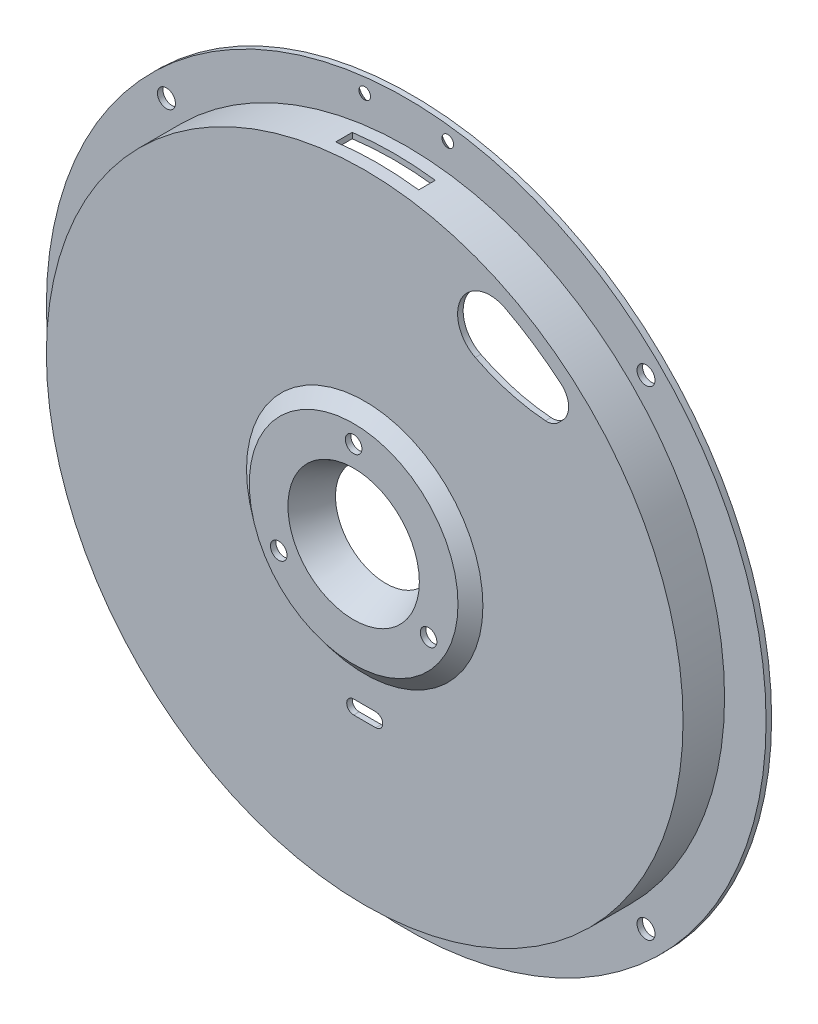
from build123d import *

# Parameters (mm, degrees)
CUT_EXTRUDE1_DEPTH                                   = 45
CUT_EXTRUDE2_DEPTH                                   = 10
SKETCH5_W                                            = 30
SKETCH5_H                                            = 6
CUT_EXTRUDE3_DEPTH                                   = 32
HOLE_SIZE_BY_CROSS_RECESS_COUNTERSUNK_SE_D           = 3.7
HOLE_SIZE_BY_CROSS_RECESS_COUNTERSUNK_SE_CSINK_D     = 8.2
HOLE_SIZE_BY_CROSS_RECESS_COUNTERSUNK_SE_CSINK_ANGLE = 90
SKETCH8_R                                            = 3.25
CUT_EXTRUDE4_DEPTH                                   = 186.04323819
CIRPATTERN1_COUNT                                    = 4
SKETCH9_R                                            = 3
CUT_EXTRUDE5_DEPTH                                   = 28
CIRPATTERN2_COUNT                                    = 3


with BuildPart() as part:
    # Sketch1 → Revolve1 (revolve)
    with BuildSketch(Plane(origin=(0, 0, 0), x_dir=(1, 0, 0), z_dir=(0, 1, 0)), mode=Mode.PRIVATE) as revolve1_sk:
        Polygon((-115, 15), (-130, 15), (-130, 17), (-113, 17), (-113, 2), (-67.400598844, 2), (-42, 2), (-37, -2), (-25, -2), (-20, 8.5), (-18.194278962, 7.640132839), (-23.737199362, -4), (-37.701562119, -4), (-42.701562119, 0), (-115, 0), align=None)
    revolve(revolve1_sk.sketch.rotate(Axis((0, 0, 0), (0, 0, -1)), 180), axis=Axis((0, 0, 0), (0, 0, -1)))

    # Sketch3 → Cut-Extrude1 (cut)
    with BuildSketch(Plane(origin=(0, 0, -17), x_dir=(-1, 0, 0), z_dir=(0, 0, -1))):
        with BuildLine():
            Line((-69.977392836, 70.947139279), (-71.467016668, 72.43676311))
            ThreePointArc((-71.467016668, 72.43676311), (-73.65767572, 78.041003905), (-71.024689008, 83.451538346))
            ThreePointArc((-71.024689008, 83.451538346), (-61.250096658, 90.868538892), (-50.7076021, 97.146306107))
            ThreePointArc((-50.7076021, 97.146306107), (-34.862231231, 92.134081811), (-39.938869953, 76.309230795))
            ThreePointArc((-39.938869953, 76.309230795), (-52.260986787, 71.486832981), (-65.295075938, 69.205911249))
            ThreePointArc((-65.295075938, 69.205911249), (-67.826068353, 69.566044861), (-69.977392836, 70.947139279))
        make_face()
    extrude(amount=-CUT_EXTRUDE1_DEPTH, mode=Mode.SUBTRACT)

    # Sketch4 → Cut-Extrude2 (cut)
    with BuildSketch(Plane(origin=(0, 0, -2), x_dir=(-1, 0, 0), z_dir=(0, 0, -1))):
        with BuildLine():
            Line((-4, -52.5), (4, -52.5))
            ThreePointArc((4, -52.5), (6.5, -55), (4, -57.5))
            Line((4, -57.5), (-4, -57.5))
            ThreePointArc((-4, -57.5), (-6.5, -55), (-4, -52.5))
        make_face()
    extrude(amount=-CUT_EXTRUDE2_DEPTH, mode=Mode.SUBTRACT)

    # Sketch5 → Cut-Extrude3 (cut)
    with BuildSketch(Plane(origin=(0, 140, 0), x_dir=(1, 0, 0), z_dir=(0, 1, 0))):
        with Locations((0, 7.5)):
            Rectangle(SKETCH5_W, SKETCH5_H)
    extrude(amount=-CUT_EXTRUDE3_DEPTH, mode=Mode.SUBTRACT)

    # Hole size by cross-recess countersunk self-tapping screw type1 (through all)
    with Locations(Plane(origin=(15, 124, -17), x_dir=(-1, 0, 0), z_dir=(0, 0, -1))):
        with Locations((0, 0), (30, 0)):
            CounterSinkHole(HOLE_SIZE_BY_CROSS_RECESS_COUNTERSUNK_SE_D / 2, HOLE_SIZE_BY_CROSS_RECESS_COUNTERSUNK_SE_CSINK_D / 2, counter_sink_angle=HOLE_SIZE_BY_CROSS_RECESS_COUNTERSUNK_SE_CSINK_ANGLE)

    # Sketch8 → Cut-Extrude4 (cut, through all)
    with BuildSketch(Plane(origin=(0, 0, -17), x_dir=(-1, 0, 0), z_dir=(0, 0, -1))):
        with Locations((86.620580695, 86.620580695)):
            Circle(SKETCH8_R)
    cut_extrude4 = extrude(amount=-CUT_EXTRUDE4_DEPTH, mode=Mode.SUBTRACT)

    # CirPattern1: Cut-Extrude4 ×4 about axis
    cirpattern1_axis = Axis((0, 0, 0), (0, 0, 1))
    for i in range(1, CIRPATTERN1_COUNT):
        add(cut_extrude4.rotate(cirpattern1_axis, i * 360 / CIRPATTERN1_COUNT), mode=Mode.SUBTRACT)

    # Sketch9 → Cut-Extrude5 (cut)
    with BuildSketch(Plane(origin=(0, 0, 2), x_dir=(-1, 0, 0), z_dir=(0, 0, -1))):
        with Locations((0, 31.25)):
            Circle(SKETCH9_R)
    cut_extrude5 = extrude(amount=-CUT_EXTRUDE5_DEPTH, mode=Mode.SUBTRACT)

    # CirPattern2: Cut-Extrude5 ×3 about axis
    cirpattern2_axis = Axis((0, 0, 0), (0, 0, 1))
    for i in range(1, CIRPATTERN2_COUNT):
        add(cut_extrude5.rotate(cirpattern2_axis, i * 360 / CIRPATTERN2_COUNT), mode=Mode.SUBTRACT)


solid = part.part
